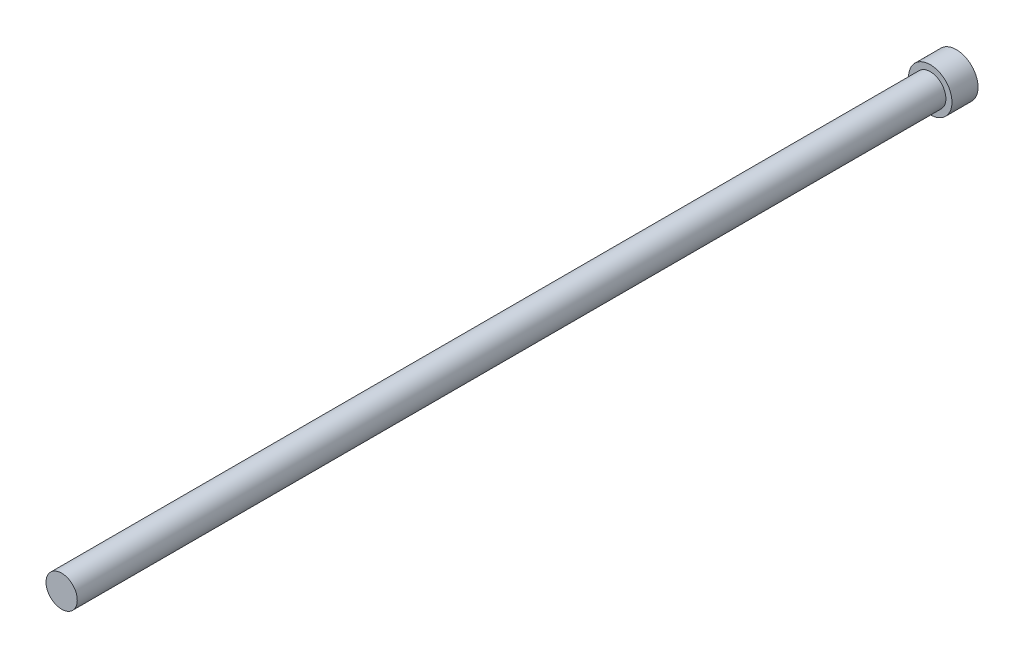
SolidWorks part; units mm, degrees
ref_plane "Front Plane" through (0, 0, 0) normal (0, 0, 1) x (1, 0, 0)
ref_plane "Top Plane" through (0, 0, 0) normal (0, 1, 0) x (1, 0, 0)
ref_plane "Right Plane" through (0, 0, 0) normal (1, 0, 0) x (0, 0, -1)
sketch "Sketch1" plane through (0, 0, 0) normal (0, 0, 1) x (1, 0, 0)
  circle A0 centre (0, 0) radius 9
  dimension "D1" = 18
extrude "Boss-Extrude1" add sketch "Sketch1" along normal blind 500
sketch "Sketch2" plane through (0, 0, 0) normal (0, 0, -1) x (-1, 0, 0)
  circle A0 centre (0, 0) radius 12.5
  dimension "D1" = 25
extrude "Boss-Extrude2" add sketch "Sketch2" along normal blind 15
